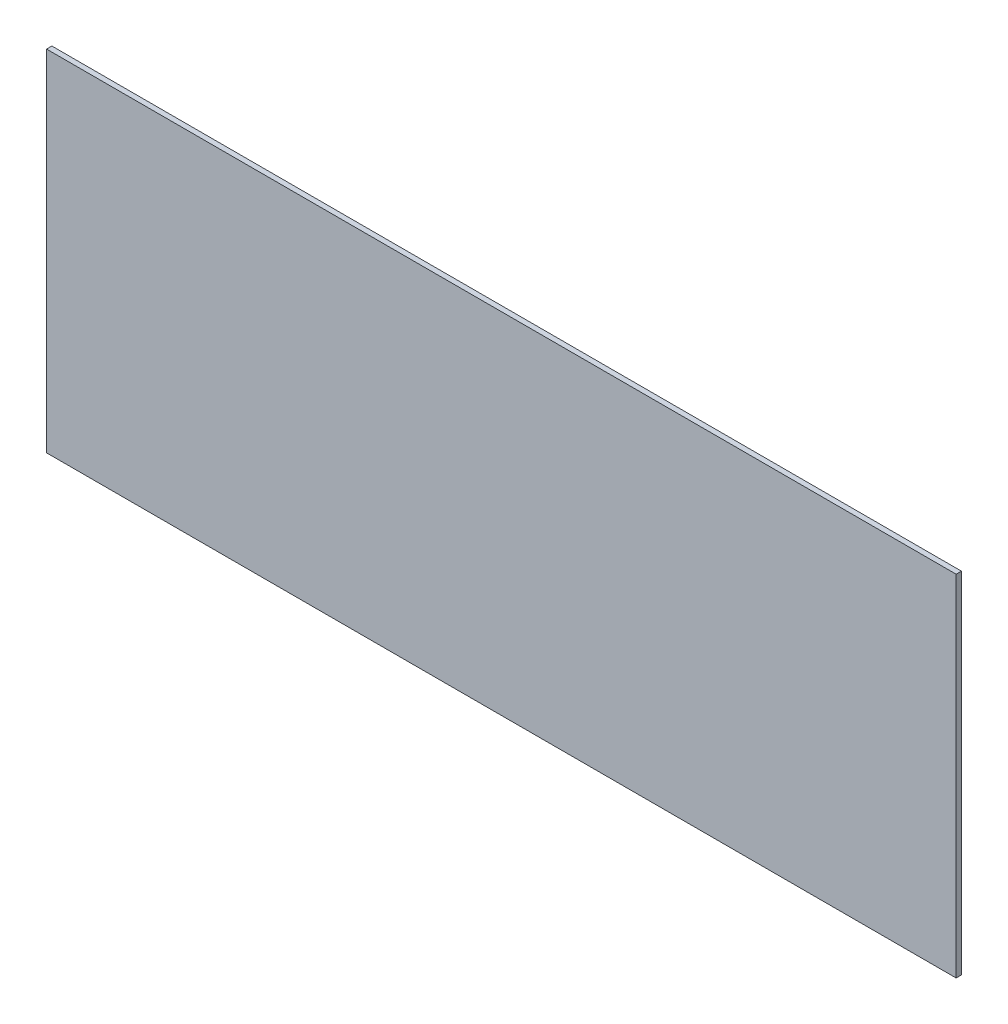
SolidWorks part; units mm, degrees
ref_plane "Frontal" through (0, 0, 0) normal (0, 0, 1) x (1, 0, 0)
ref_plane "Superior" through (0, 0, 0) normal (0, 1, 0) x (1, 0, 0)
ref_plane "Direito" through (0, 0, 0) normal (1, 0, 0) x (0, 0, -1)
sketch "Sketch1" plane through (0, 0, 0) normal (0, 0, 1) x (1, 0, 0)
  line L1 (-257.5, 99) -> (257.5, 99)
  line L2 (-257.5, 99) -> (-257.5, -99)
  line L3 (-257.5, -99) -> (257.5, -99)
  line L4 (257.5, 99) -> (257.5, -99)
  line L5 (-257.5, 99) -> (257.5, -99) construction
  line L6 (-257.5, -99) -> (257.5, 99) construction
  point P0 (0, 0)
  dimension "D1" = 198
  dimension "D2" = 515
extrude "Boss-Extrude1" add sketch "Sketch1" along normal blind 3
